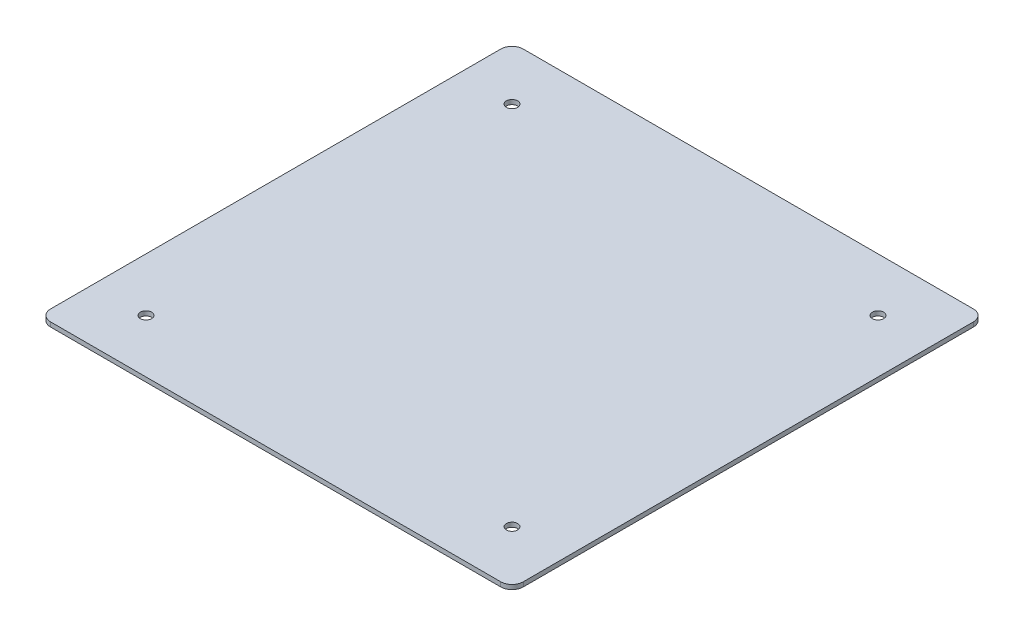
SolidWorks part; units mm, degrees
ref_plane "前视" through (0, 0, 0) normal (0, 0, 1) x (1, 0, 0)
ref_plane "上视" through (0, 0, 0) normal (0, 1, 0) x (1, 0, 0)
ref_plane "右视" through (0, 0, 0) normal (1, 0, 0) x (0, 0, -1)
sketch "草图1" plane through (0, 0, 0) normal (0, 1, 0) x (1, 0, 0)
  line L1 (-105, 105) -> (105, 105)
  line L2 (-105, 105) -> (-105, -105)
  line L3 (-105, -105) -> (105, -105)
  line L4 (105, 105) -> (105, -105)
  line L5 (-105, 105) -> (105, -105) construction
  line L6 (-105, -105) -> (105, 105) construction
  point P0 (0, 0)
  dimension "D1" = 210
  dimension "D2" = 210
extrude "凸台-拉伸1" add sketch "草图1" along normal blind 2
hole_wizard "Ø5.0 (5) 直径孔1" positions "草图3" profile "草图2" hole size "Ø5.0" standard "Gb" end condition through all
sketch "草图3" plane through (0, 2, 0) normal (0, 1, 0) x (1, 0, 0)
  line L0 (0, 0) -> (0, 111.7967) construction
  line L2 (0, 0) -> (98.5934, 98.5934) construction
  line L4 (0, 0) -> (-88.2865, 88.2865) construction
  circle A0 centre (0, 0) radius 115 construction
  point P0 (-81.3173, -81.3173)
  point P2 (-81.3173, 81.3173)
  point P4 (81.3173, 81.3173)
  point P6 (81.3173, -81.3173)
  dimension "D3" = 230
  dimension "D1" = 45
  dimension "D2" = 45
sketch "草图2" plane through (-81.3173, 2, 81.3173) normal (1, 0, 0) x (0, 0, 1)
  line L0 (0, 0) -> (0, 2)
  line L1 (0, 2) -> (2.5, 2)
  line L2 (2.5, 2) -> (2.5, 0)
  line L5 (2.5, 0) -> (0, 0)
  line L11 (0, -6.35) -> (0, 107.95) construction
  dimension "通孔孔直径" = 5
  dimension "通孔孔深度" = 2
fillet "圆角1" radius 5 4 edges at (105, 1, 105) (-105, 1, -105) (105, 1, -105) (-105, 1, 105)
